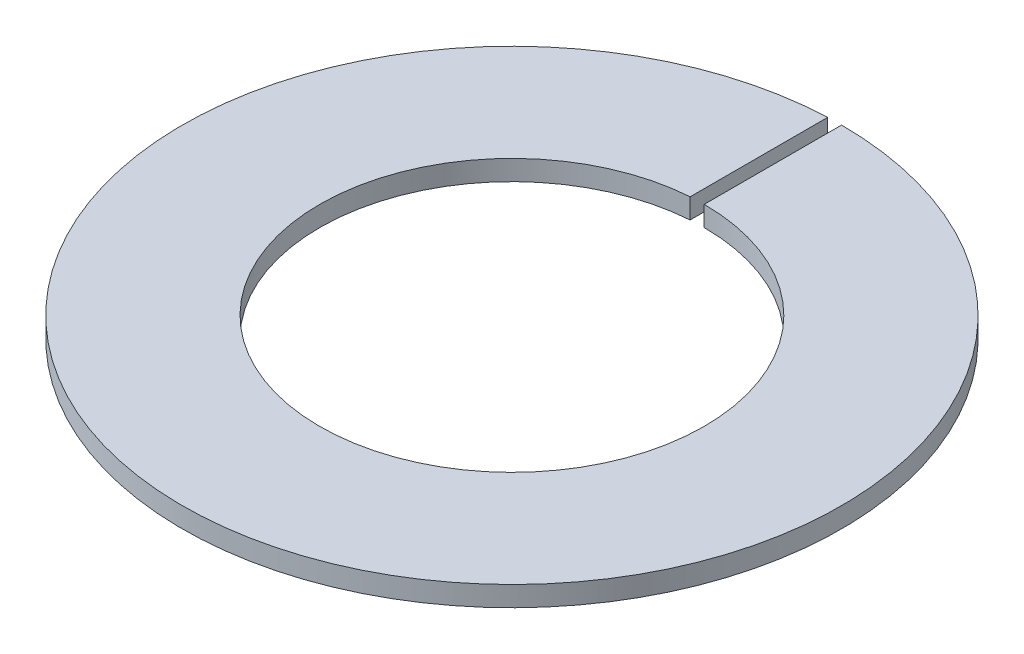
SolidWorks part; units mm, degrees
ref_plane "Front Plane" through (0, 0, 0) normal (0, 0, 1) x (1, 0, 0)
ref_plane "Top Plane" through (0, 0, 0) normal (0, 1, 0) x (1, 0, 0)
ref_plane "Right Plane" through (0, 0, 0) normal (1, 0, 0) x (0, 0, -1)
sketch "Sketch1" plane through (0, 0, 0) normal (0, 1, 0) x (1, 0, 0)
  line L0 (0, 10.5) -> (0, 18)
  line L1 (-0.7429, 17.9847) -> (-0.7429, 10.4737)
  arc A0 (-0.7429, 10.4737) -> (0, 10.5) centre (0, 0) ccw
  arc A1 (-0.7429, 17.9847) -> (0, 18) centre (0, 0) ccw
  dimension "D1" = 21
  dimension "D2" = 36
extrude "Boss-Extrude1" add sketch "Sketch1" along normal blind 1.1
